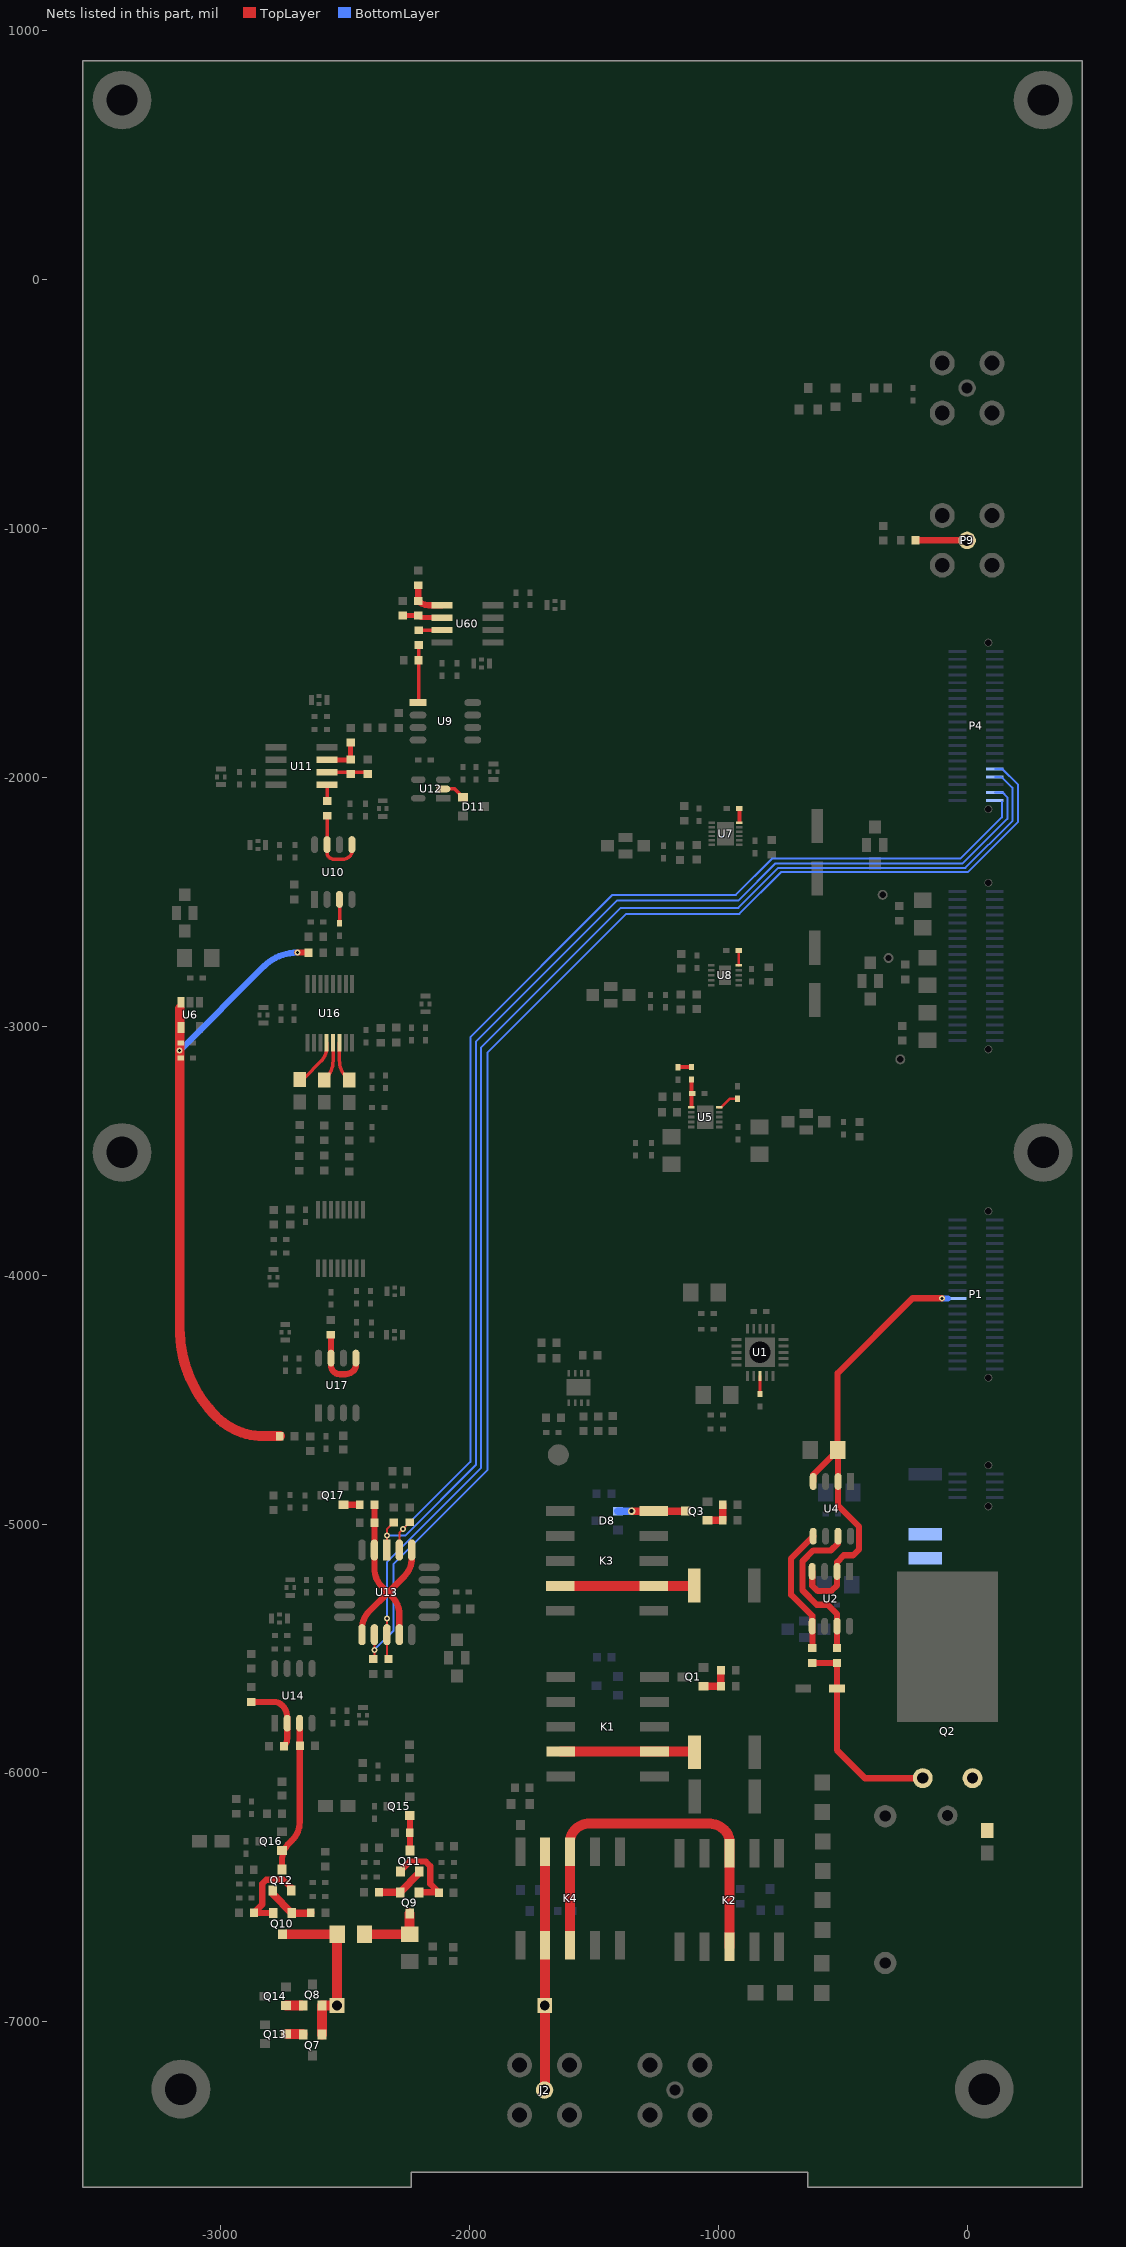
[diagram p0: the nets of this part, all layers, seen from the top]
# Altium PCB MISC109358.PcbDoc (part 6 of 7)
Units mil, origin at the board's own origin, x right, y up, seen from the top; angles counter-clockwise.
Board outline 4015.75 x 8543.31 mil, 4 copper layers (TopLayer, GND, POWER, BottomLayer), stack 33.234 mil thick; 299 components, 170 nets, 998 pads, 2318 vias.

## Via types
v1: diameter 24, hole 12, TopLayer to BottomLayer, 2184 vias
v2: diameter 20, hole 12, TopLayer to BottomLayer, 95 vias
v3: diameter 30, hole 15, TopLayer to BottomLayer, 37 vias
v4: diameter 40, hole 20, TopLayer to BottomLayer, 2 vias

## Nets (pads, with @x,y where several pads share a name; then routed paths per layer and width w, separated by ;. In a path a pad name is that pad's centre, name@x,y a point inside that pad or via, vN(x,y) a via of type N, cw(c..) or ccw(c..) an arc to the next point about the centre after c; other vN are vias at no path point) (continued)
NetD8_1: D8.1 K3.10 Q3.3 | length 274.9
  TopLayer w30: v3(-1348.5,-4947.5) Q3.3@-1129,-4947.5
  BottomLayer w30: D8.1@-1403.52,-4948.52 -1349.52,-4948.52 v3(-1348.5,-4947.5)
NetD10_2: D10.2 Q2.1 R8.1 R12.1 | length 839.7
  TopLayer w25: R12.1@-621.51,-5557.76 -523.45,-5557.76 -523.45,-5907.59 -410.34,-6020.7 Q2.1@-178.49,-6020.7
NetD11_1: D11.1 U12.2 | length 93.7
  TopLayer w14: U12.2@-2105.42,-2046.24 -2058.8,-2046.24 D11.1@-2025.52,-2079.52
NetJ2_5: J2.5 K4.2 K4.9 R18.1 | length 958.6
  TopLayer w40: J2.5@-1698,-7274 ccw(c-1704.13,-7267.87) -1695.46,-7267.87 K4.2@-1695.46,-6692.12 K4.9@-1695.46,-6316.12
NetK1_4: K1.4 K1.7 R6.1 | length 536.6
  TopLayer w40: K1.4@-1632.12,-5914.14 K1.7@-1256.12,-5914.14 R6.1@-1095.52,-5914.14
NetK2_3: K2.3 K2.8 K4.3 K4.8 | length 1558.9
  TopLayer w40: K4.3@-1595.46,-6692.12 K4.8@-1595.46,-6316.12 -1595.46,-6277.08 cw(c-1523.96,-6277.08) -1574.52,-6226.52 cw(c-1516.58,-6284.46) -1516.58,-6202.52 -1041.12,-6202.52 cw(c-1041.12,-6298.12) -973.52,-6230.52 cw(c-1017.89,-6274.89) -955.14,-6274.89 K2.3@-955.14,-6322.4 K2.8@-955.14,-6698.4
NetK3_4: K3.4 K3.7 R14.1 | length 538.6
  TopLayer w40: K3.4@-1635.12,-5248.14 K3.7@-1259.12,-5248.14 R14.1@-1096.52,-5248.14
NetL22_2: L22.2 U16.14 | length 161.5
  TopLayer w14: U16.14@-2522.19,-3066.22 -2522.19,-3135.87 ccw(c-2422.19,-3135.87) -2492.9,-3206.58 L22.2@-2483.48,-3216
NetL25_2: L25.2 U16.13 | length 158.9
  TopLayer w14: L25.2@-2582.48,-3215 -2577.07,-3209.59 ccw(c-2647.78,-3138.88) -2547.78,-3138.88 U16.13@-2547.78,-3066.22
NetL27_2: L27.2 U16.12 | length 194.7
  TopLayer w14: L27.2@-2681.48,-3214 ccw(c-2681.48,-3186.28) L27.2@-2661.89,-3205.89 ; L27.2@-2661.88,-3205.88 -2596.52,-3140.52 ccw(c-2652.41,-3084.63) -2573.37,-3084.63 U16.12@-2573.37,-3066.22
NetP9_5: P9.5 R56.2 | length 207.3
  TopLayer w25: R56.2@-207.3,-1047.18 P9.5@0,-1047.18
NetQ1_1: Q1.1 R5.1 R7.1 | length 133.2
  TopLayer w30: Q1.1@-1058.52,-5651.52 -989.48,-5651.52 -989.48,-5588 R5.1@-989,-5587.52
NetQ2_3: Q2.3 R10.2
NetQ3_1: Q3.1 R13.1 R16.1 | length 125.1
  TopLayer w30: Q3.1@-1044,-4985 -982.48,-4985 -982.14,-4984.66 R13.1@-982.14,-4921.52
NetQ7_1: Q7.1 Q8.2 Q10.3 R18.2 R38.2 | length 681.4
  TopLayer w14: Q10.3@-2751.02,-6648 -2732.52,-6648
  TopLayer w40: -2732.52,-6648 -2532.79,-6648 -2532.16,-6648.64 R18.2@-2532.16,-6934.52 Q8.2@-2592.58,-6934.52 Q7.1@-2592.58,-7050.52
NetQ7_2: Q7.2 Q13.3 | length 69.8
  TopLayer w14: Q13.3@-2736.58,-7049.02 ccw(c-2732.96,-7045.4) Q13.3@-2732.96,-7050.52 ; Q7.2@-2671.2,-7049.02 cw(c-2671.2,-7054.14) Q7.2@-2667.58,-7050.52
  TopLayer w40: Q13.3@-2732.96,-7049.02 Q7.2@-2671.2,-7049.02
NetQ8_1: Q8.1 Q14.1 | length 64.1
  TopLayer w40: Q14.1@-2737.58,-6934.52 Q8.1@-2673.52,-6934.52
NetQ9_1: Q9.1 Q11.1 R48.2 | length 345.1
  TopLayer w25: Q11.1@-2276.52,-6396.52 -2276.52,-6392.52 -2240.02,-6356.02 -2175.53,-6356.02 -2157.52,-6374.03 -2157.52,-6445.83 R48.2@-2123.83,-6479.52 ; Q9.1@-2202.52,-6479.52 R48.2@-2123.83,-6479.52 ; R48.2@-2122.83,-6480.52 R48.2@-2123.83,-6479.52
NetQ9_2: Q9.2 Q11.2 R47.1 | length 198.9
  TopLayer w30: R47.1@-2363.52,-6478.52 -2278.52,-6478.52 -2201.52,-6401.52 Q11.2@-2201.52,-6396.52
NetQ9_3: Q9.3 R37.2 R38.1 | length 265
  TopLayer w40: R38.1@-2421.52,-6648 -2240,-6648 Q9.3@-2240,-6564.54
NetQ10_1: Q10.1 Q12.1 R50.1 | length 185.3
  TopLayer w30: Q12.1@-2790.52,-6486 Q10.1@-2713.52,-6563 -2638.52,-6563 R50.1@-2637.52,-6562
NetQ10_2: Q10.2 Q12.2 R49.2 | length 357.1
  TopLayer w25: R49.2@-2866.1,-6562 -2832.52,-6528.42 -2832.52,-6445 -2816.04,-6428.52 -2747.52,-6428.52 -2715.52,-6460.52 Q12.2@-2715.52,-6473 ; R49.2@-2865.1,-6563 Q10.2@-2788.52,-6563
NetQ11_3: Q11.3 Q15.1 R51.1 | length 140
  TopLayer w25: Q11.3@-2239.02,-6311.52 Q15.1@-2239.02,-6171.5
NetQ12_3: Q12.3 Q16.1 R74.2 U14.3 | length 649.9
  TopLayer w14: Q16.1@-2753.52,-6311.48 cw(c-2754.73,-6312.69) -2753.02,-6312.69 -2753.02,-6352.4
  TopLayer w25: Q12.3@-2753.02,-6388 -2753.02,-6352.4 cw(c-2653.02,-6352.4) -2723.73,-6281.69 -2711.29,-6269.25 ccw(c-2782,-6198.54) -2682,-6198.54 U14.3@-2682,-5800
NetQ17_1: Q17.1 R64.1 | length 65.2
  TopLayer w25: Q17.1@-2505.48,-4922 -2441,-4922 R64.1@-2440.52,-4921.52
NetR1_2: R1.2 U1.3 | length 73.5
  TopLayer w12: R1.2@-831.82,-4477.52 U1.3@-831.82,-4404
NetR3_1: R3.1 R4.1
NetR8_2: R8.2 U2.7 U4.7 | length 632.5
  TopLayer w25: R8.2@-522.93,-5497.93 U2.7@-522.93,-5410.66 ; U2.7@-522.51,-5410.24 -522.51,-5361.87 -560.26,-5324.12 -603.92,-5324.12 -661.52,-5266.52 -661.52,-5149.52 -617.52,-5105.52 -547.06,-5105.52 -518.51,-5076.97 U4.7@-518.51,-5048.65
NetR12_2: R12.2 U2.5 U4.5 | length 521.9
  TopLayer w25: U2.5@-622.51,-5410.24 -622.51,-5368.53 -707.52,-5283.52 -707.52,-5137.66 U4.5@-618.51,-5048.65 ; R12.2@-621.51,-5498.45 U2.5@-621.51,-5410.24
NetR19_1: R19.1 R800.2 U5.6 | length 110.7
  TopLayer w16: R800.2@-1106.66,-3214.58 R800.2@-1107.48,-3213.76 R800.2@-1106.62,-3212.9 ; -1106.58,-3318.52 -1106.58,-3303 ; -1106.58,-3293.89 -1106.58,-3303 ; R800.2@-1106.58,-3219.34 -1106.58,-3303
NetR21_1: R21.1 U5.5 | length 87.7
  TopLayer w11: U5.5@-996.86,-3325.26 -988.26,-3325.26 -953.52,-3290.52 R21.1@-923.52,-3290.52
NetR22_1: R22.1 U7.6 | length 53.1
  TopLayer w16: U7.6@-915.52,-2178.57 R22.1@-915.52,-2125.52
NetR24_1: R24.1 U8.5 | length 59.7
  TopLayer w10: U8.5@-917.75,-2755.26 R24.1@-917.75,-2695.52
NetR26_1: R26.1 R27.1 U60.1 | length 162.9
  TopLayer w25: R26.1@-2205.52,-1227.52 R27.1@-2205.52,-1290.52 ccw(c-2163.32,-1248.32) -2163.32,-1308 U60.1@-2110.31,-1308
NetR27_2: R27.2 R35.1 U60.2 | length 160.4
  TopLayer w20: R35.1@-2268.52,-1349.83 R27.2@-2205.52,-1349.83 ccw(c-2185.79,-1330.1) -2185.79,-1358 U60.2@-2110.31,-1358
NetR29_2: R29.2 R32.1 U11.7 | length 163.3
  TopLayer w20: U11.7@-2572,-1929 -2478.48,-1929 -2478.48,-1861.31 R29.2@-2477,-1859.83
NetR30_1: R30.1 U60.3 | length 93.3
  TopLayer w14: R30.1@-2203.52,-1408.52 cw(c-2202.26,-1409.77) -2202.26,-1408 U60.3@-2110.31,-1408
NetR30_2: R30.2 R34.1 U9.1 | length 232.5
  TopLayer w14: U9.1@-2206.52,-1699.52 ccw(c-2213.76,-1692.28) -2203.52,-1692.28 R30.2@-2203.52,-1467.83
NetR31_1: R31.1 U11.5 | length 65.5
  TopLayer w14: R31.1@-2572,-2094.52 U11.5@-2572,-2029
NetR31_2: R31.2 U10.5 U10.7 | length 306.8
  TopLayer w14: R31.2@-2572,-2153.83 U10.7@-2572,-2270 -2572,-2303.87 ccw(c-2549.87,-2303.87) -2565.52,-2319.52 ccw(c-2543.79,-2297.79) -2543.79,-2328.52 -2508.08,-2328.52 ccw(c-2508.08,-2290.96) -2481.52,-2317.52 ccw(c-2504.5,-2294.54) -2472,-2294.54 U10.5@-2472,-2270
NetR32_2: R32.2 R36.1 U11.6 | length 167.6
  TopLayer w14: U11.6@-2572,-1979 -2415.04,-1979 R36.1@-2407.52,-1986.52
NetR33_2: R33.2 U10.3 | length 95
  TopLayer w14: R33.2@-2521.52,-2585.52 U10.3@-2521.52,-2490.48
NetR59_1: R59.1 R71.2 U14.2 | length 301.5
  TopLayer w25: R59.1@-2876.52,-5714.52 -2785.32,-5714.52 cw(c-2785.32,-5762.32) -2751.52,-5728.52 cw(c-2798.64,-5775.64) -2732,-5775.64 U14.2@-2732,-5800 -2732,-5860.63 cw(c-2777.1,-5860.63) R71.2@-2745.21,-5892.52
NetR64_2: R64.2 R66.2 U13.2 U13.9 U13.12 U13.19 | length 969.4
  TopLayer w25: U13.9@-2431.46,-5444.12 -2431.46,-5420.88 cw(c-2331.46,-5420.88) -2402.17,-5350.17 -2327.02,-5275.02 ; U13.2@-2381.46,-5104.12 -2381.46,-5179.16 ccw(c-2281.46,-5179.16) -2352.17,-5249.87 -2327.02,-5275.02 ; U13.2@-2381.21,-5103.86 R66.2@-2381.21,-4994.52 R64.2@-2381.21,-4921.52 ; U13.12@-2281.46,-5444.12 -2281.46,-5362 ccw(c-2381.46,-5362) -2310.75,-5291.29 -2327.02,-5275.02 ; U13.19@-2231.46,-5104.12 -2231.46,-5138.04 cw(c-2331.46,-5138.04) -2260.75,-5208.75 -2327.02,-5275.02
NetR70_1: R70.1 U17.5 U17.7 | length 291.2
  TopLayer w25: R70.1@-2557,-4239 -2556,-4240 U17.7@-2556,-4333 -2556,-4363.63 ccw(c-2523.63,-4363.63) -2546.52,-4386.52 ccw(c-2519.96,-4359.96) -2519.96,-4397.52 -2497.9,-4397.52 ccw(c-2497.9,-4353.14) -2466.52,-4384.52 ccw(c-2491.92,-4359.12) -2456,-4359.12 U17.5@-2456,-4333
NetR800_1: R800.1 R801.2 | length 55.3
  TopLayer w16: R801.2@-1162.48,-3164.52 -1161.72,-3163.76 R800.1@-1107.48,-3163.76
TT: P1.22 R9.1 U2.2 U2.4 U4.2 U4.4 | length 1857.6
  TopLayer w25: U2.4@-622.51,-5190.24 -622.51,-5247.53 -601.52,-5268.52 -545.52,-5268.52 -522.51,-5245.51 U2.2@-522.51,-5190.24 -522.51,-5152.51 -495.52,-5125.52 -458.52,-5125.52 -434,-5101 -434,-5011.04 -518.51,-4926.53 U4.2@-518.51,-4828.65 -518.51,-4703.53 R9.1@-520.52,-4701.52 ; U4.4@-618.51,-4828.65 -618.51,-4801.51 -520.52,-4703.52 R9.1@-520.52,-4701.52 ; v1(-100.52,-4092.52) -219.52,-4092.52 -520.52,-4393.52 R9.1@-520.52,-4701.52
  BottomLayer w25: v1@-100.08,-4092.96 -76.52,-4092.96
U15_IN1: P4.39 R61.1 U13.20 | length 4783.8
  TopLayer w8: U13.20@-2281.46,-5104.12 -2281.46,-5034.99 v1(-2266.99,-5020.52) R61.1@-2238.99,-4992.52
  BottomLayer w8: v1(-2266.99,-5020.52) -1996.4,-4749.93 -1996.4,-3043.4 -1425,-2472 -929.48,-2472 -784,-2326.52 -27.02,-2326.52 139.48,-2160.02 P4.39@139.48,-2096.37
U15_IN2: P4.37 R60.2 U13.1 | length 4949.8
  TopLayer w8: U13.1@-2331.46,-5104.12 v1(-2331.46,-5046.52) -2331.46,-5021.3 R60.2@-2302.99,-4992.83
  BottomLayer w8: v1(-2331.46,-5046.52) -2257.52,-5046.52 -1973.52,-4762.52 -1973.52,-3514.52 -1973.52,-3062.52 -1405,-2494 -918.48,-2494 -770,-2345.52 -18.02,-2345.52 161.48,-2166.02 161.48,-2079.52 142.41,-2060.45 P4.37@111.04,-2060.45
U15_IN3: P4.33 R65.1 U13.11 | length 5340.4
  TopLayer w8: R65.1@-2331.46,-5535.77 U13.11@-2331.46,-5444.12 v1(-2331.46,-5378.96)
  BottomLayer w8: v1@-2331.52,-5378.52 -2331.52,-5153.52 -1953.52,-4775.52 -1953.52,-3496.52 -1953.52,-3086.52 -1391,-2524 -919.48,-2524 -759,-2363.52 -7.02,-2363.52 181.48,-2175.02 181.48,-2041.08 137.85,-1997.46 P4.33@111.04,-1997.46
U15_IN4: P4.31 R69.2 U13.10 | length 5464.8
  TopLayer w8: R69.2@-2381.46,-5536.7 v1(-2381.46,-5505.52) U13.10@-2381.46,-5444.12
  BottomLayer w8: v1(-2381.46,-5505.52) -2305.52,-5429.58 -2305.52,-5160.52 -1926.52,-4781.52 -1926.52,-3606.52 -1926.52,-3104.52 -1370,-2548 -915.48,-2548 -748,-2380.52 1.98,-2380.52 203.48,-2179.02 203.48,-2027.52 141.92,-1965.96 P4.31@111.04,-1965.96
VREF: C38.2 C41.2 R28.1 R67.2 U6.3 U6.4 | length 2628.9
  TopLayer w25: v1(-2691.52,-2703.52) R28.1@-2646.52,-2703.52
  TopLayer w40: -3163.71,-2927.52 -3163.71,-3067.83 -3163.71,-4214.36 ccw(c-2664.03,-4214.36) -3017.36,-4567.68 ccw(c-2827.02,-4377.35) -2827.02,-4646.52 R67.2@-2761.83,-4646.52
  BottomLayer w25: v1(-3164.52,-3097.52) -2826.38,-2759.38 cw(c-2691.52,-2894.24) v1(-2691.52,-2703.52)
pads on no net: D2.2 D3.2 D8.2 D9.2 D11.2 K1.2 K1.5 K1.6 K1.9 K2.5 K2.6 K3.2 K3.5 K3.6 K3.9 K4.5 K4.6 P1.0 P1.1 P1.2 P1.3 P1.4 P1.7 P1.8 P1.9 P1.10 P1.13 P1.14 P1.15 P1.16 P1.25 P1.26 P1.28 P1.31 P1.32 P1.33 P1.34 P1.37 P1.38 P1.39 P1.40 P2.0 P4.0 P4.1 P4.3 P4.7 P5.0 Q5.2 Q6.2 Q7.3 Q8.3 Q13.2 Q14.2 U1.2 U1.4 U1.8 U1.10 U1.12 U1.17 U1.18 U1.19 U2.1 U2.8 U4.1 U4.8 U5.4 U7.4 U7.7 U8.4 U9.5 U9.6 U11.1 U11.2 U11.3 U12.1 U14.1 U14.5 U15.1 U15.2 U15.4 U15.5 U16.1 U16.2 U16.4 U16.5 U60.5 U60.6 U60.7

## Polygon pours and split planes (outlines as drawn)
GND on TopLayer "Bottom Layer-No Net" (solid, remove dead copper): 226,-4527 226,-6368 273,-6415 275,-6417 294,-6417 388,-6417 413,-6392 433,-6372 433,-6272 433,-4460 402,-4429 388,-4415 357,-4415 254,-4415 233,-4436 226,-4443 226,-4527
GND on TopLayer "GND_L01_P064" (solid, remove dead copper, pour order 64): -3764.06,616.82 -3882.06,498.82 -3882.06,-7776.18 -3706.06,-7952.18 485.94,-7952.18 714.94,-7723.18 714.94,-6391.18 609.94,-6286.18 0.94,-6286.18 -24.06,-6311.18 -24.06,-6606.18 -73.06,-6655.18 -444.06,-6655.18 -498.06,-6601.18 -498.06,-6054.7 -425.06,-5981.7 -425.06,-4559.18 -399.06,-4533.18 562.94,-4533.18 635.94,-4460.18 635.94,1063.82 399.94,1299.82 -3534.06,1299.82 -3764.06,1069.82
NetC47_1 on TopLayer "NETC47_1_L01_P006" (solid, remove dead copper, pour order 6): -1325.52,-2298.52 -1321.52,-2302.52 -1263.52,-2302.52 -1249.34,-2288.34 -1022.34,-2288.34 -1012.52,-2278.52 -1012.52,-2231.52 -1014.52,-2229.52 -1164.52,-2229.52 -1196.52,-2197.52 -1311.52,-2197.52 -1325.52,-2211.52
-5V on TopLayer "-5V_L01_P062" (solid, remove dead copper, pour order 62): -1560.52,-2355.52 -1541.52,-2374.52 -1457.52,-2374.52 -1420.52,-2337.52 -1420.52,-2244.52 -1438.52,-2226.52 -1522.52,-2226.52 -1560.52,-2264.52
+5V on TopLayer "+5V_L01_P060" (solid, remove dead copper, pour order 60): -1587.52,-2940.52 -1568.52,-2959.52 -1496.83,-2959.52 -1480.52,-2943.21 -1480.52,-2805.52 -1493.33,-2792.71 -1575.71,-2792.71 -1587.52,-2804.52
no net on TopLayer "NONET_L01_P058" (solid, remove dead copper, pour order 58): -3208.52,-2389.52
+5V on TopLayer "+5V_L01_P056" (solid, remove dead copper, pour order 56): -3196.52,-2481.52 -3179.52,-2498.52 -3094.04,-2498.52 -3080.52,-2485 -3080.52,-2387.52 -3090.52,-2377.52 -3187.21,-2377.52 -3196.52,-2386.83
NetQ2_3 on TopLayer "NETQ2_3_L01_P054" (solid, remove dead copper, pour order 54): -27.52,-5988.52 -27.52,-6065.52 18.48,-6111.52 18.48,-6239.52 40.48,-6261.52 154.48,-6261.52 179.48,-6236.52 179.48,-6015.52 134.48,-5970.52 -9.52,-5970.52
H5V on TopLayer "H5V_L01_P044" (solid, remove dead copper, pour order 44): -1714.52,-4957.79 -1701.79,-4970.52 -1487.52,-4970.52 -1474.52,-4957.52 -1474.52,-4909.21 -1494.21,-4889.52 -1540.52,-4889.52 -1593.52,-4836.52 -1593.52,-4683.52 -1568.52,-4658.52 -1472.52,-4658.52 -1462.52,-4648.52 -1462.52,-4615.4 -1469.4,-4608.52 -1567.52,-4608.52 -1576.52,-4599.52 -1576.52,-4541.52 -1568.52,-4533.52 -1568.52,-4499.52 -1571.52,-4496.52 -1617.6,-4496.52 -1648.52,-4527.44 -1648.52,-4598.52 -1654.52,-4604.52 -1654.52,-4647.52 -1714.52,-4707.52
H12V on TopLayer "H12V_L01_P042" (solid, remove dead copper, pour order 42): -995.52,-4623.52 -986.52,-4632.52 -939.52,-4632.52 -926.31,-4619.31 -926.31,-4574.75 -907.08,-4555.52 -825.52,-4555.52 -818.52,-4548.52 -818.52,-4519.52 -824.52,-4513.52 -856.52,-4513.52 -876.52,-4493.52 -876.52,-4386.52 -879,-4384.04 -895.91,-4384.04 -905.52,-4374.43 -905.52,-4357.52 -907.52,-4355.52 -963.52,-4355.52 -981,-4373 -981,-4520 -995.52,-4534.52
NetC39_1 on TopLayer "NETC39_1_L01_P028" (solid, remove dead copper, pour order 28): -3216.52,-2841.52 -3194.52,-2863.52 -3148.52,-2863.52 -3136.52,-2875.52 -3136.52,-2920.52 -3132.52,-2924.52 -3069.47,-2924.52 -3063.52,-2918.57 -3063.52,-2868.52 -3108.52,-2823.52 -3108.52,-2602.52 -3120.52,-2590.52 -3195.52,-2590.52 -3216.52,-2611.52
A12V on TopLayer "A12V_L01_P024" (solid, remove dead copper, pour order 24): -1375.52,-3461.52 -1354.52,-3482.52 -1141.52,-3482.52 -1094.96,-3435.96 -1094.96,-3380.08 -1096.52,-3378.52 -1146.52,-3378.52 -1162.52,-3394.52 -1353.52,-3394.52 -1375.52,-3416.52
NetC32_1 on TopLayer "NETC32_1_L01_P022" (solid, remove dead copper, pour order 22): -1010.52,-3408.52 -1001.52,-3417.52 -897.52,-3417.52 -873.52,-3441.52 -717.52,-3441.52 -694.52,-3418.52 -694.52,-3348.52 -710.52,-3332.52 -919.52,-3332.52 -946.22,-3359.22 -1008.22,-3359.22 -1010.52,-3361.52
12.4V on TopLayer "12.4V_L01_P016" (solid, remove dead copper, pour order 16): -600.52,-3406.52 -595.52,-3411.52 -538.52,-3411.52 -524.52,-3397.52 -242.52,-3397.52 -116.52,-3271.52 -116.52,-3038.52 -134.52,-3020.52 -201.52,-3020.52 -220.52,-3039.52 -314.52,-3039.52 -364.02,-3089.02 -364.02,-3192.02 -414.52,-3242.52 -547.94,-3242.52 -600.52,-3295.09
NetC58_1 on TopLayer "NETC58_1_L01_P014" (solid, remove dead copper, pour order 14): -1385.52,-2897.52 -1378.52,-2904.52 -1315.52,-2904.52 -1299.52,-2888.52 -1031.52,-2888.52 -1015.52,-2872.52 -1015.52,-2812.52 -1019.08,-2808.95 -1186.08,-2808.95 -1210.52,-2784.52 -1359.52,-2784.52 -1385.52,-2810.52
NetC59_2 on TopLayer "NETC59_2_L01_P012" (solid, remove dead copper, pour order 12): -930.52,-2906.52 -857.52,-2979.52 -383.52,-2979.52 -344.52,-2940.52 -344.52,-2871.52 -352.52,-2863.52 -491.77,-2863.52 -530.77,-2824.52 -730.52,-2824.52 -748.52,-2806.52 -876.52,-2806.52 -893.52,-2789.52 -928.69,-2789.52 -930.52,-2791.35
A6V on TopLayer "A6V_L01_P008" (solid, remove dead copper, pour order 8): -430.52,-2758.52 -417.52,-2771.52 -215.52,-2771.52 -202.52,-2758.52 -127.52,-2758.52 -116.52,-2747.52 -116.52,-2700.52 -134.52,-2682.52 -250.52,-2682.52 -280.52,-2652.52 -412.52,-2652.52 -430.52,-2670.52
NetC45_2 on TopLayer "NETC45_2_L01_P004" (solid, remove dead copper, pour order 4): -1004.52,-2273.52 -1001.52,-2276.52 -869.75,-2276.52 -861.75,-2268.52 -574.02,-2268.52 -531.02,-2225.52 -347.52,-2225.52 -340.52,-2218.52 -340.52,-2116.52 -378.52,-2078.52 -631.52,-2078.52 -747.52,-2194.52 -927.76,-2194.52 -928.52,-2195.28 -928.52,-2203.52 -927.52,-2204.52 -899.52,-2204.52 -896.52,-2207.52 -896.52,-2225.52 -901.1,-2230.1 -933.94,-2230.1 -937.52,-2226.52 -937.52,-2177.52 -939.52,-2175.52 -1002.52,-2175.52 -1004.52,-2177.52
-5.4V on TopLayer "-5.4V_L01_P000" (solid, remove dead copper, pour order 0): -414.52,-2472.52 -354.52,-2532.52 -151.52,-2532.52 -137.52,-2518.52 -137.52,-2414.52 -233.52,-2318.52 -395.52,-2318.52 -414.52,-2337.52
A6V on TopLayer "Bottom Layer-No Net" (solid, remove dead copper, pour order 1000): -1668.52,-4268.52 -1668.52,-4376.52 -1649.52,-4395.52 -1637.52,-4407.52 -1602.52,-4407.52 -1570.52,-4407.52 -1569.52,-4406.52 -1568.52,-4405.52 -1568.52,-4403.52 -1568.52,-4259.52 -1580.52,-4247.52 -1584.52,-4243.52 -1604.52,-4243.52 -1657.52,-4243.52 -1664.52,-4250.52 -1668.52,-4254.52 -1668.52,-4268.52
12.4V on TopLayer "Bottom Layer-No Net" (solid, remove dead copper, pour order 1001): -1033.52,-4093.52 -1033.52,-4229 -1023.52,-4239 -998,-4264.52 -939.52,-4264.52 -907.52,-4264.52 -906.52,-4263.52 -905.52,-4262.52 -905.52,-4259.52 -905.52,-4243.52 -901.52,-4239.52 -897.52,-4235.52 -887.52,-4235.52 -879.52,-4235.52 -877.52,-4233.52 -876.52,-4232.52 -876.52,-4231.52 -876.52,-4178.41 -885.41,-4169.52 -898.52,-4156.41 -898.52,-4110.52 -898.52,-4040.52 -911.52,-4027.52 -917.52,-4021.52 -945.52,-4021.52 -1021.52,-4021.52 -1029.52,-4029.52 -1033.52,-4033.52 -1033.52,-4093.52
GND on BottomLayer "Bottom Layer-No Net" (solid, remove dead copper): 226,-4512 226,-6389 253,-6416 263,-6426 283,-6426 407,-6426 414,-6419 433,-6400 433,-6259 433,-4495 404,-4466 394,-4456 370,-4456 267,-4456 261,-4462 226,-4497 226,-4512
A6V on BottomLayer "Bottom Layer-No Net" (solid, remove dead copper): -1668,-4232 -1668,-4377.04 -1649.52,-4395.52 -1642.04,-4403 -1603,-4403 -1504,-4403 -1496,-4395 -1492,-4391 -1492,-4369 -1492,-4353.61 -1498.08,-4347.53 -1503.61,-4342 -1518,-4342 -1533,-4342 -1538,-4337 -1542,-4333 -1542,-4317 -1542,-4171 -1433,-4062 -1263,-3892 -1136,-3892 -1004,-3892 -1000,-3892 -800,-3692 -754,-3692 -719,-3692 -706,-3679 -682,-3655 -682,-3444 -682,-3238 -609,-3165 -494,-3050 -494,-2912 -494,-2803 -464,-2773 -438,-2747 -362,-2747 -340,-2747 -289,-2798 -277,-2810 45,-2810 147,-2810 151.48,-2805.52 151.48,-2709.52 146.48,-2704.52 145.96,-2704 89,-2704 -113.04,-2704 -134.52,-2682.52 -135.04,-2682 -213,-2682 -228,-2682 -259,-2651 -264,-2646 -324,-2646 -482,-2646 -548,-2712 -618,-2782 -618,-2884 -618,-2971 -718,-3071 -781,-3134 -781,-3465 -781,-3556 -810,-3585 -822,-3597 -855,-3597 -868,-3597 -918,-3647 -1044,-3773 -1184,-3773 -1324,-3773 -1487,-3936 -1668,-4117 -1668,-4232
12.4V on BottomLayer "Bottom Layer-No Net" (solid, remove dead copper): -961,-4029 -961,-4039 -961,-4195 -953,-4203 -943,-4213 -888,-4213 -819,-4213 -810,-4204 -805,-4199 -805,-4184 -805,-4165 -812,-4158 -817,-4153 -836,-4153 -843,-4153 -849,-4147 -854,-4142 -854,-4111 -854,-3998 -818,-3962 -759,-3903 -635,-3903 -446,-3903 -287,-3744 -126,-3583 -126,-3298 -126,-3192 0,-3066 2,-3064 80,-3064 147,-3064 150,-3061 152,-3059 152,-3050 152,-2930 149,-2927 147,-2925 139,-2925 -72,-2925 -126,-2979 -204.52,-3057.52 -261.52,-3057.52 -291.52,-3057.52 -320,-3086 -320,-3160 -320,-3495 -452,-3627 -556,-3731 -657,-3731 -783,-3731 -892,-3840 -961,-3909 -961,-4029
NetC18_1 on BottomLayer "NETC18_1_L04_P052" (solid, remove dead copper, pour order 52): -237.52,-5639.52 -162.52,-5714.52 30.48,-5714.52 86.48,-5770.52 86.48,-6090.52 58.48,-6118.52 -357.52,-6118.52 -383.52,-6144.52 -383.52,-6240.52 -363.52,-6260.52 135.48,-6260.52 179.48,-6216.52 179.48,-5479.11 44.89,-5344.52 -227.52,-5344.52 -237.52,-5354.52
GND on BottomLayer "GND_L04_P066" (solid, remove dead copper, pour order 66): -3764.97,617 -3882.97,499 -3882.97,-7776 -3706.97,-7952 485.03,-7952 714.03,-7723 714.03,-6391 609.03,-6286 0.03,-6286 -24.97,-6311 -24.97,-6606 -73.97,-6655 -444.97,-6655 -498.97,-6601 -498.97,-6054.52 -425.97,-5981.52 -425.97,-4559 -399.97,-4533 562.03,-4533 635.03,-4460 635.03,1064 399.03,1300 -3534.97,1300 -3764.97,1070
NetR3_1 on BottomLayer "NETR3_1_L04_P050" (solid, remove dead copper, pour order 50): -251.52,-5153.8 -240.8,-5164.52 -90.52,-5164.52 -76.52,-5150.52 -76.52,-5024.52 -89.52,-5011.52 -237.8,-5011.52 -251.52,-5025.24
HT on BottomLayer "HT_L04_P048" (solid, remove dead copper, pour order 48): -245.55,-4751.52 -245.55,-4822.33 -240.36,-4827.52 -91.52,-4827.52 -82.52,-4836.52 -82.52,-4892.39 -72.39,-4902.52 -6.52,-4902.52 -2.52,-4898.52 -2.52,-4775.52 -35.52,-4742.52 -236.55,-4742.52
H5V on BottomLayer "H5V_L04_P046" (solid, remove dead copper, pour order 46): -1550.52,-4985.52 -1528.69,-5007.35 -1475.47,-5007.35 -1467.52,-4999.4 -1467.52,-4859.65 -1472.65,-4854.52 -1532.13,-4854.52 -1550.52,-4872.91
A6V on BottomLayer "A6V_L04_P010" (solid, remove dead copper, pour order 10): -342.52,-2745.52 -277.52,-2810.52 146.48,-2810.52 151.48,-2805.52 151.48,-2709.52 146.48,-2704.52 -112.52,-2704.52 -134.52,-2682.52 -333.52,-2682.52 -342.52,-2691.52
-5.4V on BottomLayer "-5.4V_L04_P002" (solid, remove dead copper, pour order 2): -277.52,-2476.52 -163.52,-2590.52 148.48,-2590.52 152.48,-2586.52 152.48,-2458.52 146.48,-2452.52 -77.52,-2452.52 -123.1,-2406.94 -263.94,-2406.94 -277.52,-2420.52
GND on GND (split plane): 442.65,-7643.9 -620.2,-7643.9 -620.2,-7604.94 -620.59,-7601.02 -621.73,-7597.25 -623.59,-7593.78 -626.09,-7590.73 -629.13,-7588.24 -632.61,-7586.38 -636.38,-7585.23 -640.3,-7584.85 -2233.7,-7584.85 -2237.62,-7585.23 -2241.39,-7586.38 -2244.87,-7588.24 -2247.91,-7590.73 -2250.41,-7593.78 -2252.27,-7597.25 -2253.41,-7601.02 -2253.8,-7604.94 -2253.8,-7643.9 -3532.9,-7643.9 -3532.9,859.21 442.65,859.21
GND on POWER (split plane): 442.65,-7643.9 -620.2,-7643.9 -620.2,-7604.94 -620.59,-7601.02 -621.73,-7597.25 -623.59,-7593.78 -626.09,-7590.73 -629.13,-7588.24 -632.61,-7586.38 -636.38,-7585.23 -640.3,-7584.85 -2233.7,-7584.85 -2237.62,-7585.23 -2241.39,-7586.38 -2244.87,-7588.24 -2247.91,-7590.73 -2250.41,-7593.78 -2252.27,-7597.25 -2253.41,-7601.02 -2253.8,-7604.94 -2253.8,-7643.9 -3532.9,-7643.9 -3532.9,-6711.61 -2164.52,-6711.61 -2161.91,-6711.26 -2159.48,-6710.25 -2157.39,-6708.65 -1450.39,-6001.65 -1448.78,-5999.56 -1447.78,-5997.13 -1447.43,-5994.52 -1447.43,-3291.7 -843.87,-2688.13 -842.26,-2686.04 -841.76,-2684.83 -841.26,-2683.61 -840.91,-2681 -840.91,-1574 -841.26,-1571.39 -841.97,-1569.67 -842.26,-1568.96 -843.87,-1566.87 -1229.35,-1181.39 -1231.44,-1179.78 -1233.87,-1178.78 -1236.48,-1178.43 -3532.9,-1178.43 -3532.9,859.21 442.65,859.21